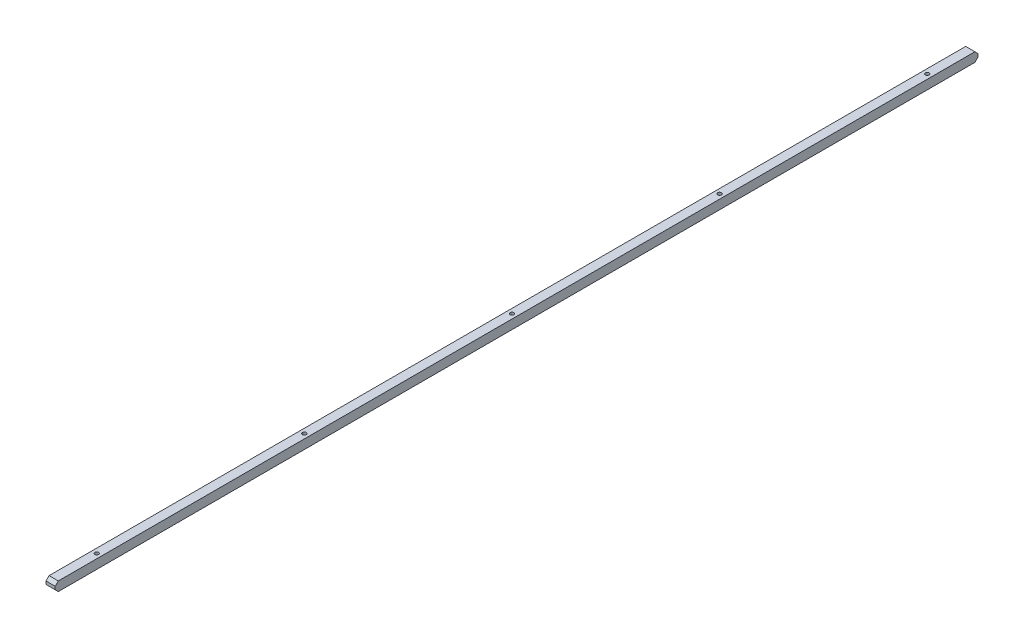
SolidWorks part; units mm, degrees
material "AISI 1045 钢，冷拔"
ref_plane "前视基准面" through (0, 0, 0) normal (0, 0, 1) x (1, 0, 0)
ref_plane "上视基准面" through (0, 0, 0) normal (0, 1, 0) x (1, 0, 0)
ref_plane "右视基准面" through (0, 0, 0) normal (1, 0, 0) x (0, 0, -1)
sketch "草图1" plane through (0, 0, 0) normal (0, 0, 1) x (1, 0, 0)
  line L1 (-3, 3) -> (3, 3)
  line L2 (-3, 3) -> (-3, -3)
  line L3 (-3, -3) -> (3, -3)
  line L4 (3, 3) -> (3, -3)
  line L5 (-3, 3) -> (3, -3) construction
  line L6 (-3, -3) -> (3, 3) construction
  point P0 (0, 0)
  dimension "D1" = 6
extrude "凸台-拉伸1" add sketch "草图1" along normal blind 600
sketch "草图2" plane through (0, 3, 0) normal (0, 1, 0) x (1, 0, 0)
  line L0 (0, 0) -> (0, -165) construction
  line L1 (0, -165) -> (0, -300) construction
  line L2 (0, -300) -> (0, -435) construction
  line L3 (0, -435) -> (0, -600) construction
  line L4 (3, -600) -> (-3, -600) construction
  line L5 (0, -165) -> (0, -30) construction
  line L6 (0, -435) -> (0, -570) construction
  dimension "D1" = 135
  dimension "D2" = 135
  dimension "D3" = 135
hole_wizard "M3 螺纹孔1" positions "3D草图1" profile "草图3" tap size "M3" standard "GB" end condition through all
sketch3d "3D草图1"
  point P0 (0, 3, 165)
  point P3 (0, 3, 300)
  point P6 (0, 3, 435)
  point P9 (0, 3, 570)
  point P12 (0, 3, 30)
sketch "草图3" plane through (0, 3, 165) normal (1, 0, 0) x (0, 0, 1)
  line L0 (0, 0) -> (0, 6)
  line L1 (0, 6) -> (1.25, 6)
  line L2 (1.25, 6) -> (1.25, 0)
  line L5 (1.25, 0) -> (0, 0)
  line L11 (0, -6.35) -> (0, 107.95) construction
  dimension "通孔螺纹孔钻头直径" = 2.5
  dimension "通孔螺纹孔钻头深度" = 6
cosmetic thread "孔螺蚊线1" parameters "D2"=3
cosmetic thread "孔螺蚊线2" parameters "D2"=3
cosmetic thread "孔螺蚊线3" parameters "D2"=3
cosmetic thread "孔螺蚊线4" parameters "D2"=3
cosmetic thread "孔螺蚊线5" parameters "D2"=3
chamfer "倒角1" distance 2 angle 45 4 edges at (0, -3, 0) (0, 3, 0) (0, -3, 600) (0, 3, 600)
